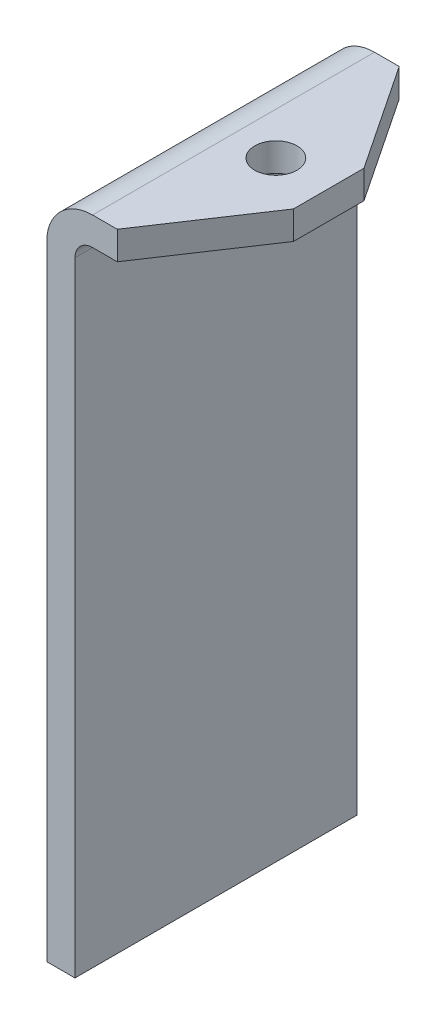
SolidWorks part; units mm, degrees
material "1023 Carbon steel plate (SS)"
ref_plane "Front Plane" through (0, 0, 0) normal (0, 0, 1) x (1, 0, 0)
ref_plane "Top Plane" through (0, 0, 0) normal (0, 1, 0) x (1, 0, 0)
ref_plane "Right Plane" through (0, 0, 0) normal (1, 0, 0) x (0, 0, -1)
sketch "Sketch1" plane through (0, 0, 0) normal (0, 0, 1) x (1, 0, 0)
  line L0 (0, 0) -> (-27, 0)
  line L1 (-40, -13) -> (-40, -190)
  line L2 (0, -8) -> (-27, -8)
  line L3 (-32, -13) -> (-32, -190)
  line L4 (0, 0) -> (0, -8)
  line L5 (-40, -190) -> (-32, -190)
  arc A0 (-27, 0) -> (-40, -13) centre (-27, -13) ccw
  arc A1 (-27, -8) -> (-32, -13) centre (-27, -13) ccw
  point P6 (-40, 0)
  dimension "D3" = 13
  dimension "D1" = 40
  dimension "D2" = 190
  dimension "D4" = 8
extrude "Boss-Extrude1" add sketch "Sketch1" along normal blind 80 contours L5 L3 A1 L2 L4 L0 A0 L1
sketch "Sketch2" plane through (0, 0, 0) normal (0, 1, 0) x (1, 0, 0)
  line L0 (-20, 0) -> (0, -30)
  line L1 (0, 0) -> (-27, 0) construction
  line L2 (0, -80) -> (0, 0) construction
  line L3 (0, -30) -> (0, 0)
  line L4 (0, 0) -> (-20, 0)
  line L5 (0, -40) -> (-14.0007, -40) construction
  line L6 (0, -50) -> (0, -80)
  line L7 (-20, -80) -> (0, -50)
  line L8 (0, -80) -> (-20, -80)
  line L9 (-40, -80) -> (-40, 0) construction
  circle A0 centre (-15, -40) radius 6
  dimension "D3" = 25
  dimension "D4" = 12
  dimension "D1" = 20
  dimension "D2" = 30
extrude "Cut-Extrude1" cut sketch "Sketch2" against normal blind 12 contours L6 L8 L7 | L4 L0 L3 | A0
